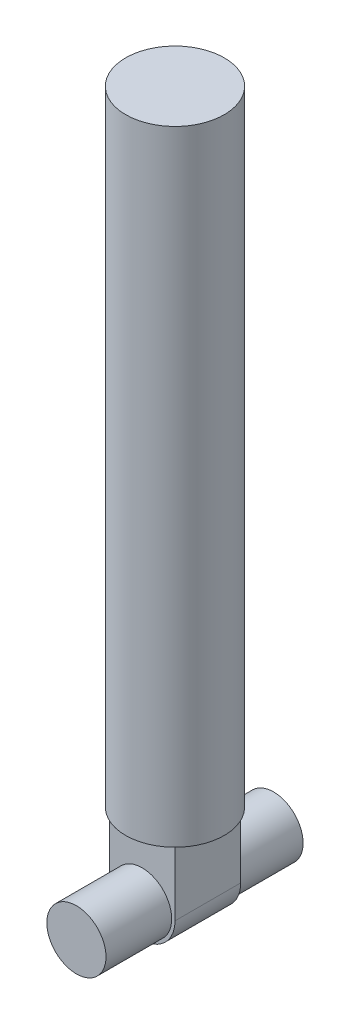
from build123d import *

# Parameters (mm, degrees)
SKETCH_1_R           = 15
EXTRUDE_1_DEPTH      = 190
EXTRUDE_2_DEPTH      = 10
EXTRUDE_2_DEPTH_BACK = 10
EXTRUDE_3_DEPTH      = 20
EXTRUDE_3_DEPTH_BACK = 40
SKETCH_3_R           = 9


with BuildPart() as part:
    # 草图1 → 凸台-拉伸1 (new body)
    with BuildSketch(Plane(origin=(0, 0, 0), x_dir=(1, 0, 0), z_dir=(0, 1, 0))):
        with Locations(Location((0, 0, 0), (0, 0, 270))):
            Circle(SKETCH_1_R)
    extrude(amount=EXTRUDE_1_DEPTH)

    # 草图2 → 凸台-拉伸2 (add, two sides: drawn at the far end of the back side and taken through both)
    with BuildSketch(Plane.XY.offset(-EXTRUDE_2_DEPTH_BACK)):
        with BuildLine():
            Line((10, 0), (10, -20))
            ThreePointArc((10, -20), (0, -30), (-10, -20))
            Line((-10, -20), (-10, 0))
            ThreePointArc((-10, 0), (0, 10), (10, 0))
        make_face()
    extrude(amount=EXTRUDE_2_DEPTH + EXTRUDE_2_DEPTH_BACK)

    # 草图3 → 凸台-拉伸3 (add, two sides: drawn at the far end of the back side and taken through both)
    with BuildSketch(Plane.XY.offset(10).offset(-EXTRUDE_3_DEPTH_BACK)):
        with Locations((0, -20)):
            Circle(SKETCH_3_R)
    extrude(amount=EXTRUDE_3_DEPTH + EXTRUDE_3_DEPTH_BACK)


solid = part.part
